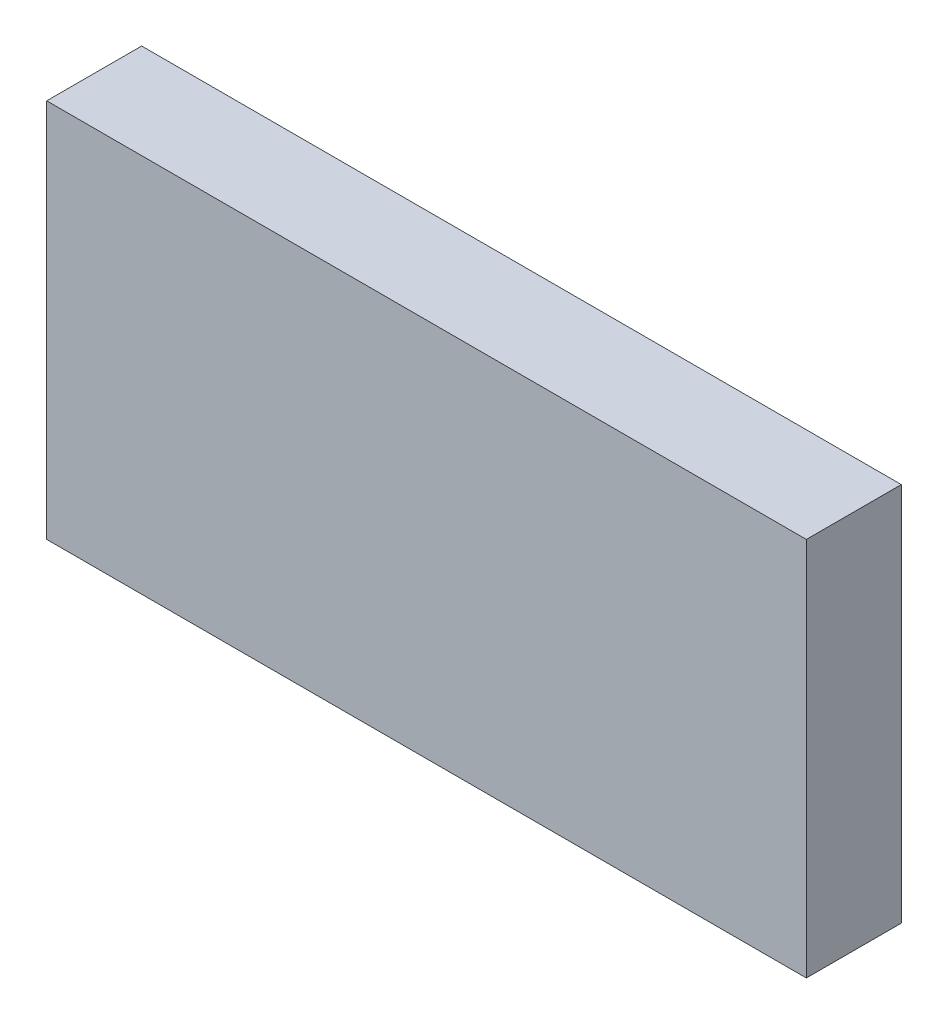
from build123d import *

# Parameters (mm, degrees)
SKETCH1_W           = 240
SKETCH1_H           = 120
BOSS_EXTRUDE1_DEPTH = 30


with BuildPart() as part:
    # Sketch1 → Boss-Extrude1 (new body)
    with BuildSketch(Plane.XY):
        with Locations((88.34299394, 39.34299394)):
            Rectangle(SKETCH1_W, SKETCH1_H)
    extrude(amount=BOSS_EXTRUDE1_DEPTH)


solid = part.part
